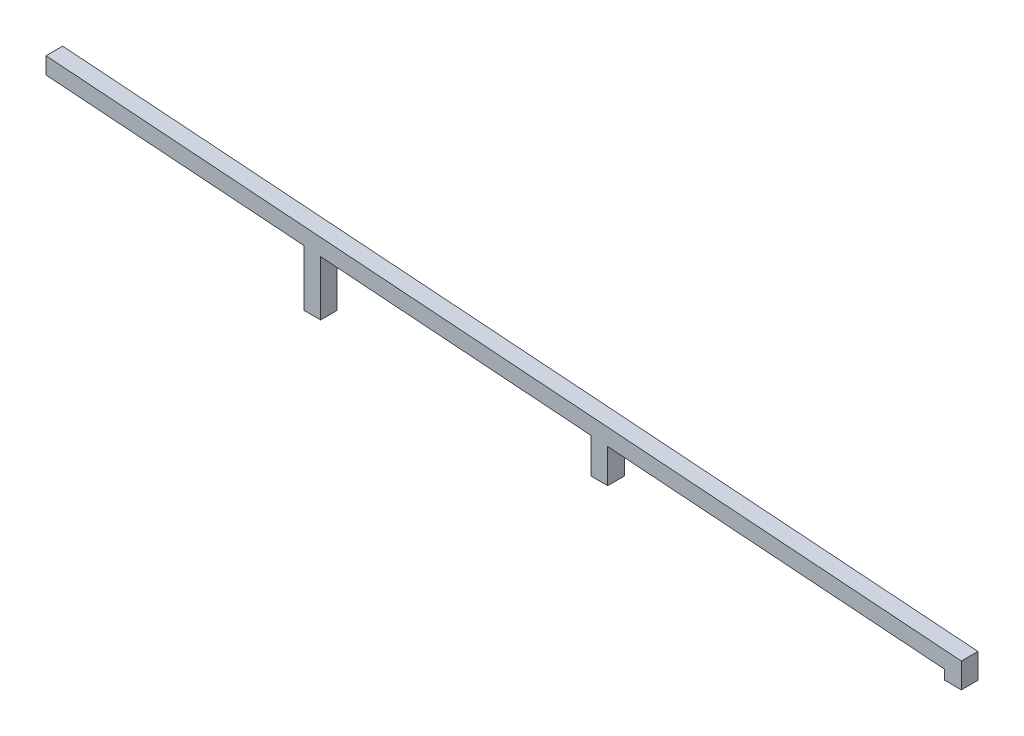
from build123d import *

# Parameters (mm, degrees)
BOSS_EXTRUDE1_DEPTH = 40


with BuildPart() as part:
    # Sketch1 → Boss-Extrude1 (new body)
    with BuildSketch(Plane.XY):
        Polygon((2200, 0), (2200, 60), (0, 220), (0, 179.894354388), (620, 134.803445298), (620, 0), (660, 0), (660, 131.894354388), (1310, 84.621627116), (1310, 0), (1350, 0), (1350, 81.712536207), (2160, 22.803445298), (2160, 0), align=None)
    extrude(amount=BOSS_EXTRUDE1_DEPTH)


solid = part.part
